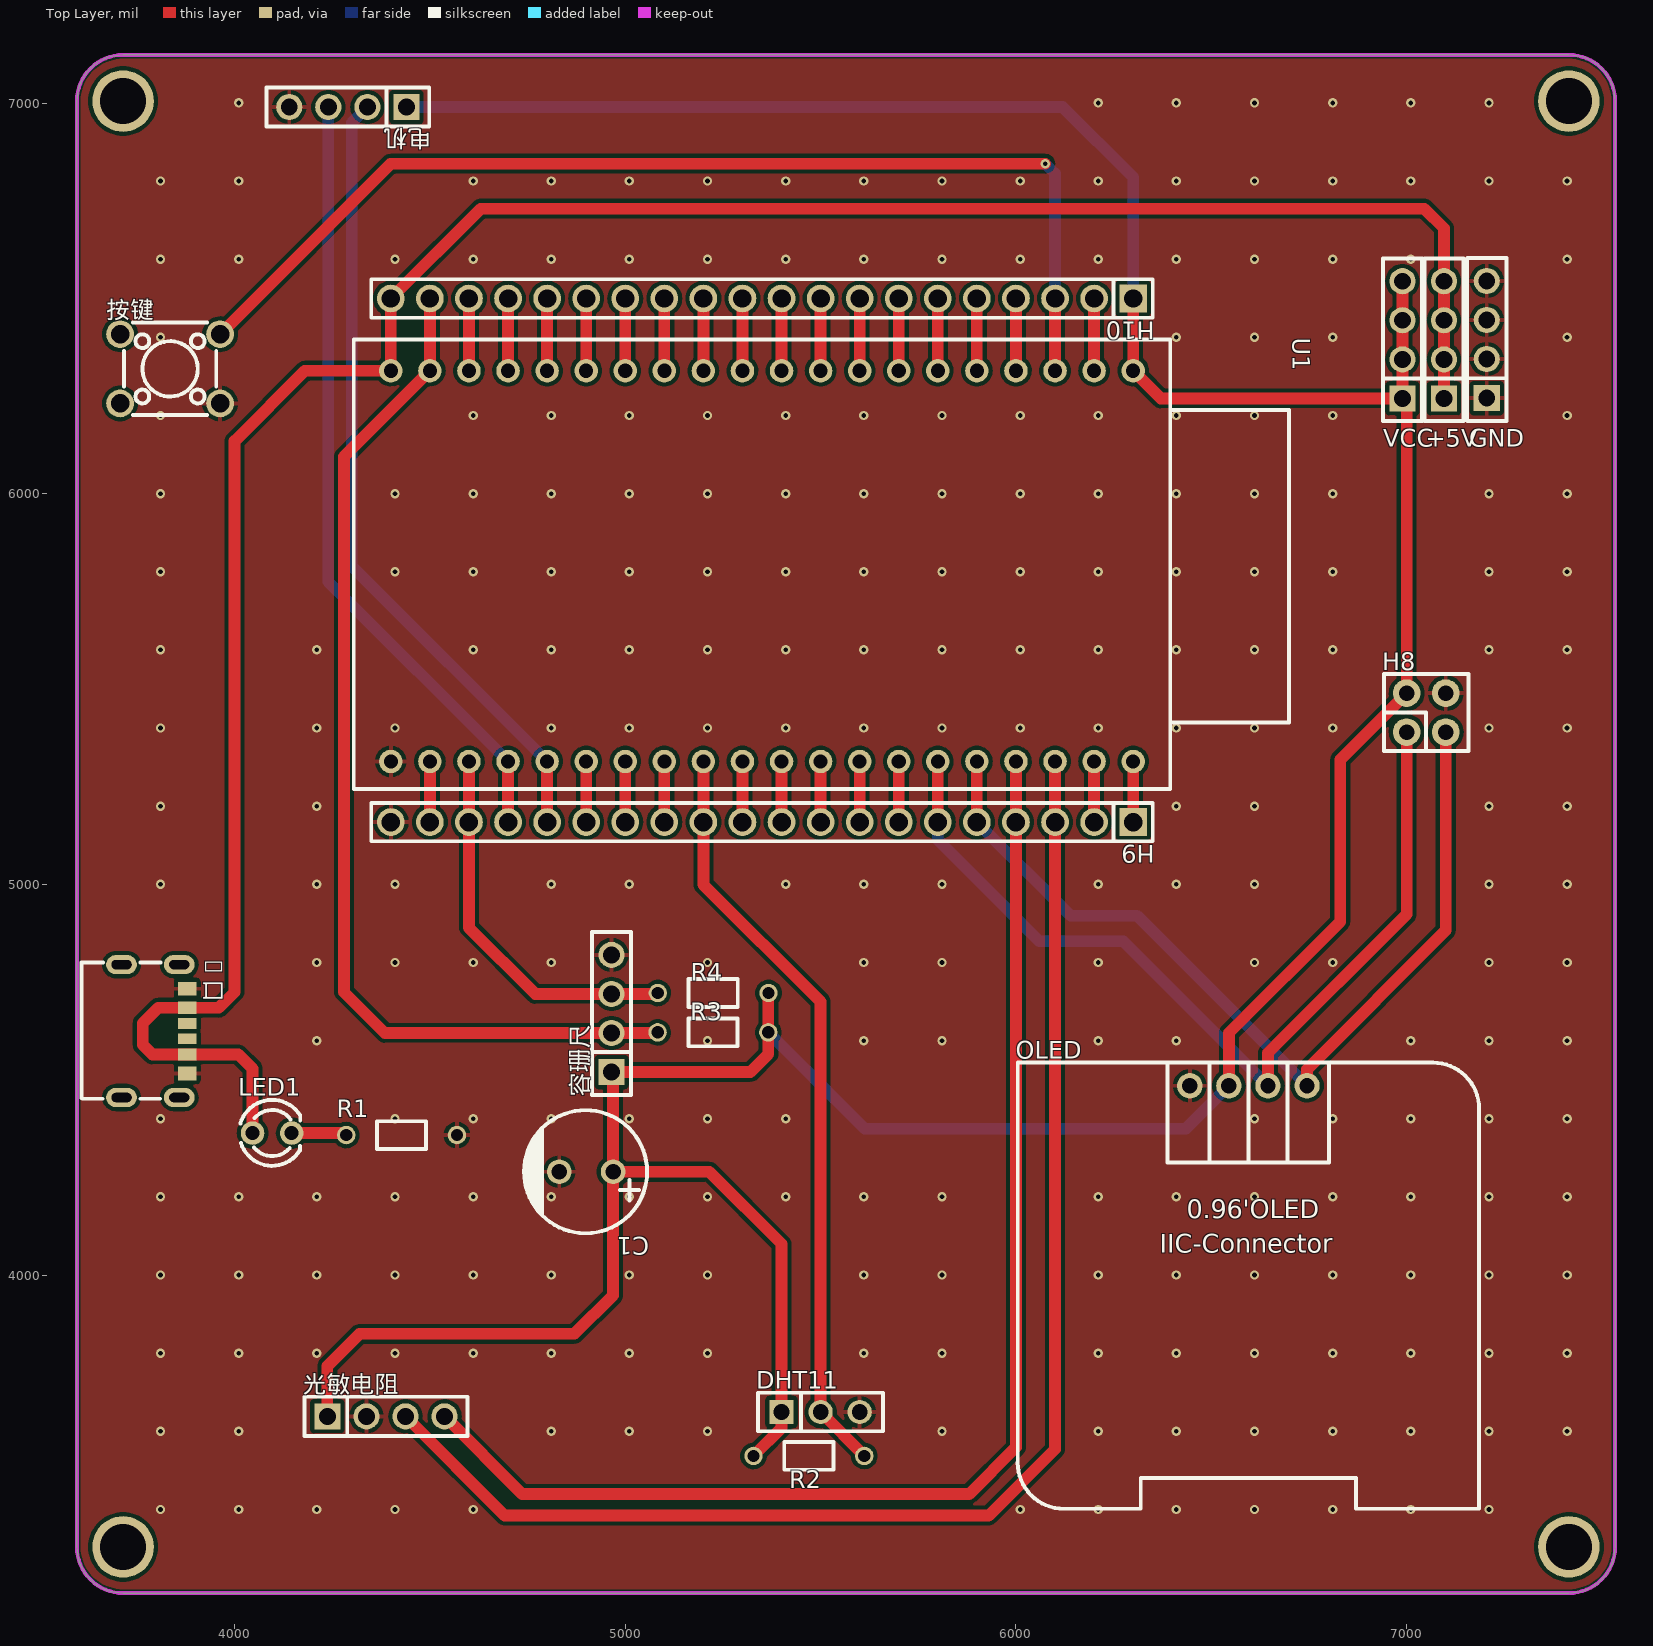
[diagram p0: Top Layer view]
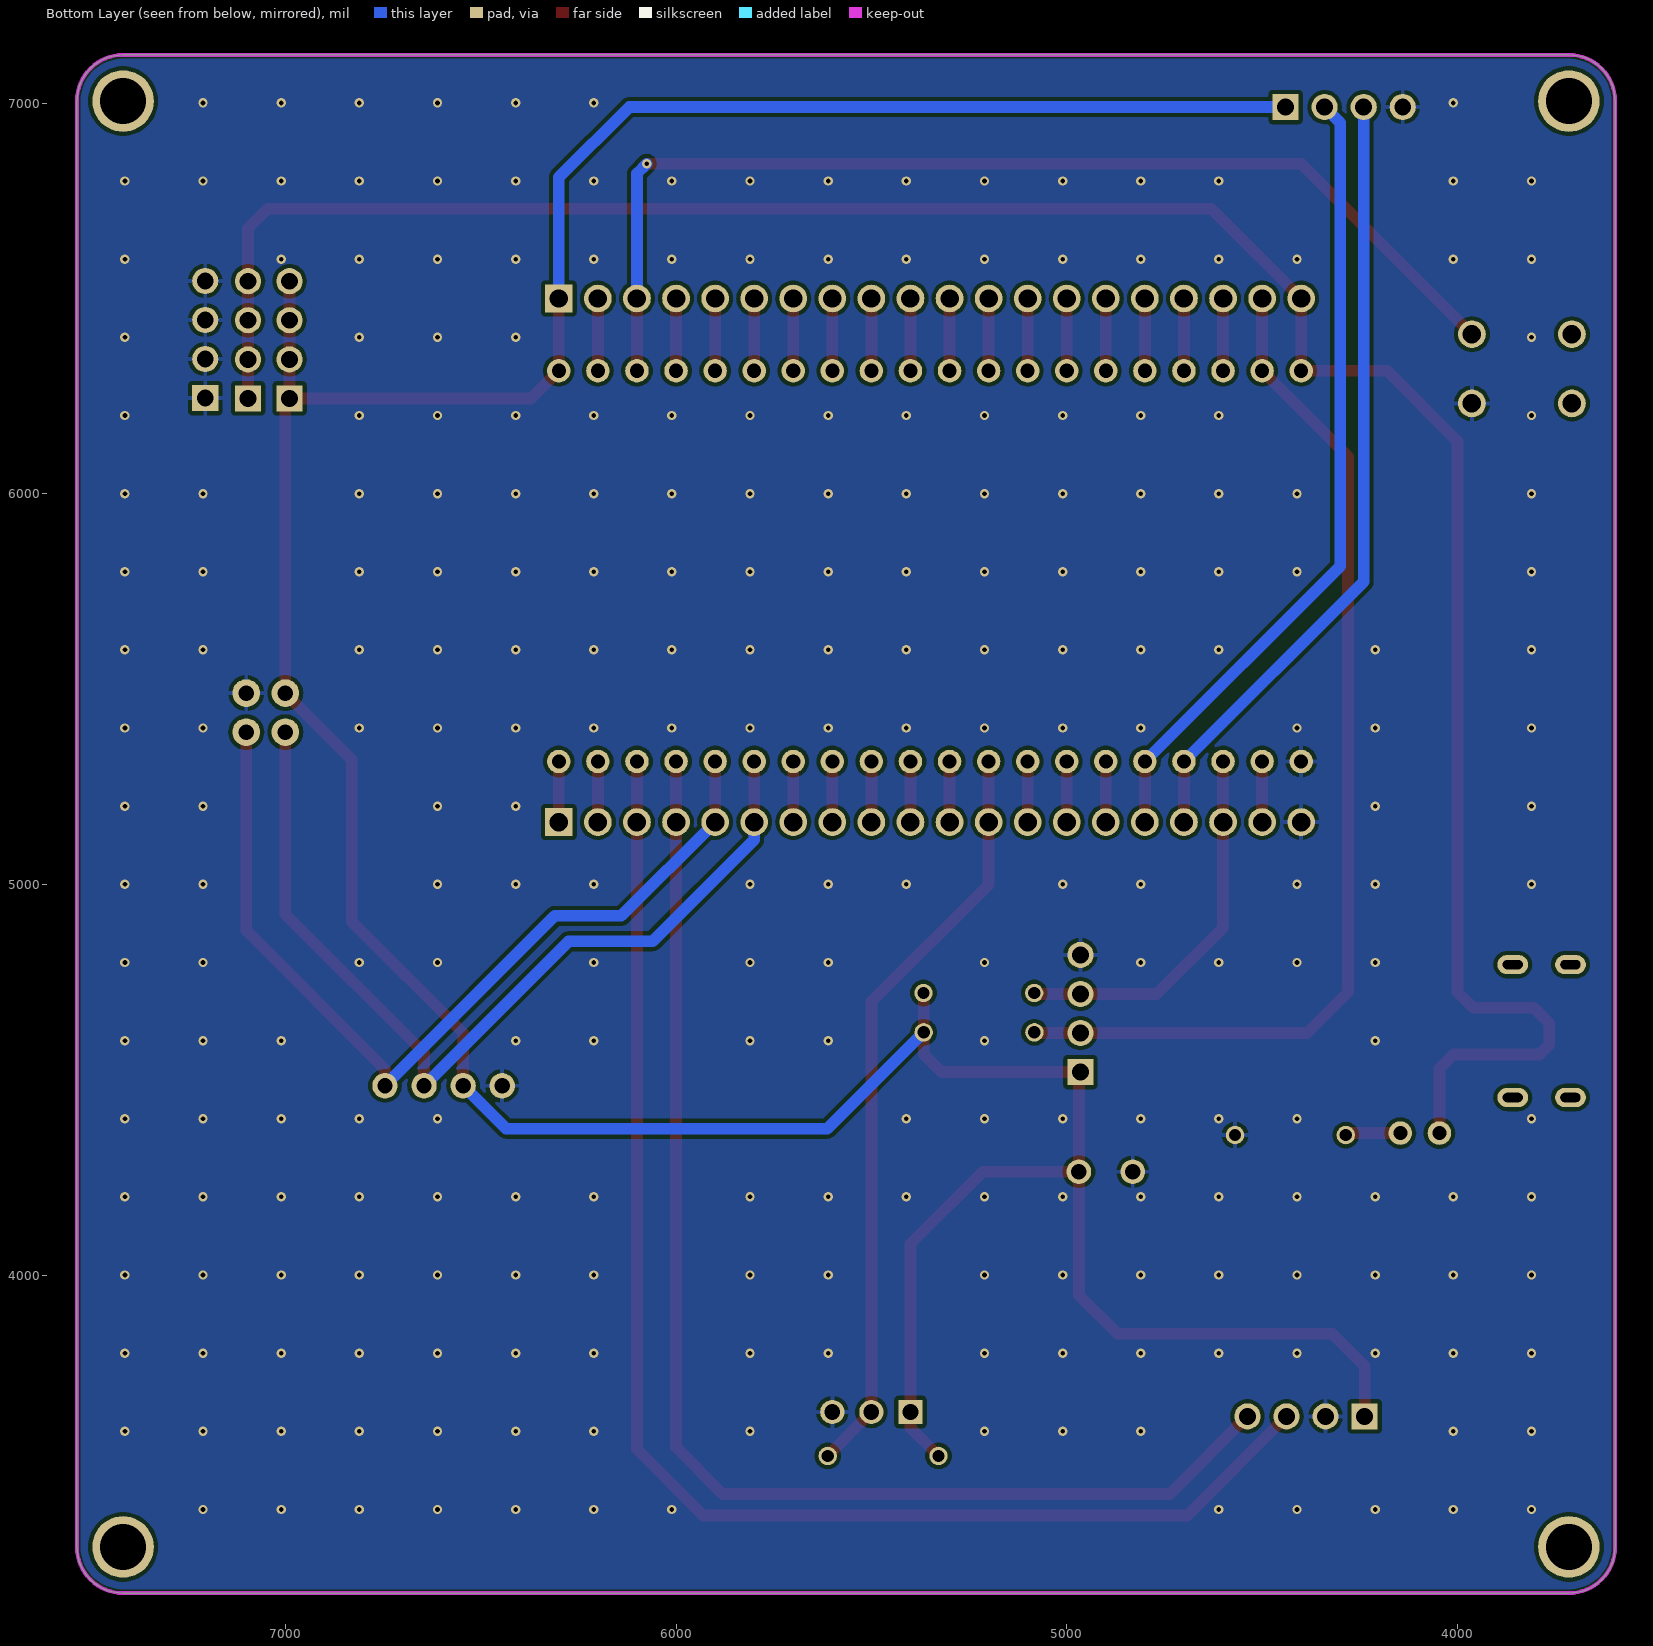
[diagram p1: Bottom Layer view, seen from below]
# Altium PCB MISC51152.pcbdoc
Units mil, origin at the board's own origin, x right, y up, seen from the top; angles counter-clockwise.
Board outline 3937.01 x 3937.01 mil, 2 copper layers (Top Layer, Bottom Layer), stack 62.206 mil thick; 20 components, 41 nets, 145 pads, 254 vias.

## Layer stack, top to bottom
Top Solder Mask Layer: solder mask 0.394, Dk 3.3
Top Layer: signal copper 1.379
Dielectric1: surface 59.449, FR4, Dk 4.5
Bottom Layer: signal copper 1.378
Bottom Solder Mask Layer: solder mask 0.394, Dk 3.3

## Board outline
3714.61,7123.5 ccw(c3714.61,7005.39) 3596.5,7005.39 3596.5,3304.61 ccw(c3714.61,3304.61) 3714.61,3186.5 7415.39,3186.5 ccw(c7415.39,3304.61) 7533.5,3304.61 7533.5,7005.39 ccw(c7415.39,7005.39) 7415.39,7123.5 3714.61,7123.5

## Design rules (kind name [scope] priority, off if disabled: settings)
BoardOutlineClearance copperThickness2oz_1 [All] p2 off: genericclearance=7.99 ignorepadtopadclearanceinfootprint=FALSE except(0: Arc-SplitContinuation Track-SplitContinuation SMDPad-SplitContinuation THPad-SplitContinuation Via-SplitContinuation Fill-SplitContinuation Region-SplitContinuation Poly-SplitContinuation Text-SplitContinuation Hole-SplitContinuation; 5.98: Arc-CutoutEdge Track-CutoutEdge SMDPad-CutoutEdge THPad-CutoutEdge Via-CutoutEdge Text-CutoutEdge; 6.9: Hole-OutlineEdge Hole-CutoutEdge; 10: Poly-OutlineEdge Poly-CutoutEdge; 11.81: Arc-OutlineEdge Track-OutlineEdge SMDPad-OutlineEdge THPad-OutlineEdge Via-OutlineEdge Fill-OutlineEdge Region-OutlineEdge Text-OutlineEdge Fill-CutoutEdge Region-CutoutEdge)
BoardOutlineClearance Plane_innerPlane_1 [All] p4 off: genericclearance=4.02 ignorepadtopadclearanceinfootprint=FALSE except(0: Arc-SplitContinuation Track-SplitContinuation SMDPad-SplitContinuation THPad-SplitContinuation Via-SplitContinuation Fill-SplitContinuation Region-SplitContinuation Poly-SplitContinuation Text-SplitContinuation Hole-SplitContinuation; 5.98: Arc-CutoutEdge Track-CutoutEdge SMDPad-CutoutEdge THPad-CutoutEdge Via-CutoutEdge Text-CutoutEdge; 6.9: Hole-OutlineEdge Hole-CutoutEdge; 10: Poly-OutlineEdge Poly-CutoutEdge; 11.81: Arc-OutlineEdge Track-OutlineEdge SMDPad-OutlineEdge THPad-OutlineEdge Via-OutlineEdge Fill-OutlineEdge Region-OutlineEdge Text-OutlineEdge Fill-CutoutEdge Region-CutoutEdge)
BoardOutlineClearance Copper_copperRegion_1 [All] p6 off: genericclearance=4.02 ignorepadtopadclearanceinfootprint=FALSE except(0: Arc-SplitContinuation Track-SplitContinuation SMDPad-SplitContinuation THPad-SplitContinuation Via-SplitContinuation Fill-SplitContinuation Region-SplitContinuation Poly-SplitContinuation Text-SplitContinuation Hole-SplitContinuation; 5.98: Arc-CutoutEdge Track-CutoutEdge SMDPad-CutoutEdge THPad-CutoutEdge Via-CutoutEdge Text-CutoutEdge; 6.9: Hole-OutlineEdge Hole-CutoutEdge; 10: Poly-OutlineEdge Poly-CutoutEdge; 11.81: Arc-OutlineEdge Track-OutlineEdge SMDPad-OutlineEdge THPad-OutlineEdge Via-OutlineEdge Fill-OutlineEdge Region-OutlineEdge Text-OutlineEdge Fill-CutoutEdge Region-CutoutEdge)
BoardOutlineClearance Copper_copperRegion_copperThickness1oz_1 [All] p8 off: genericclearance=4.02 ignorepadtopadclearanceinfootprint=FALSE except(0: Arc-SplitContinuation Track-SplitContinuation SMDPad-SplitContinuation THPad-SplitContinuation Via-SplitContinuation Fill-SplitContinuation Region-SplitContinuation Poly-SplitContinuation Text-SplitContinuation Hole-SplitContinuation; 5.98: Arc-CutoutEdge Track-CutoutEdge SMDPad-CutoutEdge THPad-CutoutEdge Via-CutoutEdge Text-CutoutEdge; 6.9: Hole-OutlineEdge Hole-CutoutEdge; 10: Poly-OutlineEdge Poly-CutoutEdge; 11.81: Arc-OutlineEdge Track-OutlineEdge SMDPad-OutlineEdge THPad-OutlineEdge Via-OutlineEdge Fill-OutlineEdge Region-OutlineEdge Text-OutlineEdge Fill-CutoutEdge Region-CutoutEdge)
BoardOutlineClearance Copper_copperRegion_Copper_copperRegion_1 [All] p10 off: genericclearance=4.02 ignorepadtopadclearanceinfootprint=FALSE except(0: Arc-SplitContinuation Track-SplitContinuation SMDPad-SplitContinuation THPad-SplitContinuation Via-SplitContinuation Fill-SplitContinuation Region-SplitContinuation Poly-SplitContinuation Text-SplitContinuation Hole-SplitContinuation; 5.98: Arc-CutoutEdge Track-CutoutEdge SMDPad-CutoutEdge THPad-CutoutEdge Via-CutoutEdge Text-CutoutEdge; 6.9: Hole-OutlineEdge Hole-CutoutEdge; 10: Poly-OutlineEdge Poly-CutoutEdge; 11.81: Arc-OutlineEdge Track-OutlineEdge SMDPad-OutlineEdge THPad-OutlineEdge Via-OutlineEdge Fill-OutlineEdge Region-OutlineEdge Text-OutlineEdge Fill-CutoutEdge Region-CutoutEdge)
BoardOutlineClearance copperThickness1oz_1 [All] p12: genericclearance=4.02 ignorepadtopadclearanceinfootprint=FALSE except(0: Arc-SplitContinuation Track-SplitContinuation SMDPad-SplitContinuation THPad-SplitContinuation Via-SplitContinuation Fill-SplitContinuation Region-SplitContinuation Poly-SplitContinuation Text-SplitContinuation Hole-SplitContinuation; 5.98: Arc-CutoutEdge Track-CutoutEdge SMDPad-CutoutEdge THPad-CutoutEdge Via-CutoutEdge Text-CutoutEdge; 6.9: Hole-OutlineEdge Hole-CutoutEdge; 10: Poly-OutlineEdge Poly-CutoutEdge; 11.81: Arc-OutlineEdge Track-OutlineEdge SMDPad-OutlineEdge THPad-OutlineEdge Via-OutlineEdge Fill-OutlineEdge Region-OutlineEdge Text-OutlineEdge Fill-CutoutEdge Region-CutoutEdge)
Clearance copperThickness2oz [All] p1 off: gap=7.99 ignorepadtopadclearanceinfootprint=FALSE except(5.98: SMDPad-Track SMDPad-SMDPad THPad-Track SMDPad-THPad THPad-THPad Track-Via SMDPad-Via THPad-Via Via-Via Fill-SMDPad Region-SMDPad Fill-THPad Region-THPad Fill-Via Region-Via Fill-Fill Fill-Region Region-Region Arc-Track Arc-SMDPad Arc-THPad Arc-Via Fill-Arc Region-Arc Arc-Arc Text-Track SMDPad-Text Text-THPad Text-Via Fill-Text Region-Text Arc-Text Text-Text; 6.9: Hole-Track Hole-SMDPad Hole-THPad Hole-Via Fill-Hole Region-Hole Hole-Arc Hole-Text; 10: Poly-Track Poly-SMDPad Poly-THPad Poly-Via Poly-Fill Poly-Region Poly-Poly Poly-Arc Poly-Text Poly-Hole; 11.81: Fill-Track Region-Track)
Clearance Plane_innerPlane [All] p3 off: gap=4.02 ignorepadtopadclearanceinfootprint=FALSE except(5.98: SMDPad-Track SMDPad-SMDPad THPad-Track SMDPad-THPad THPad-THPad Track-Via SMDPad-Via THPad-Via Via-Via Fill-SMDPad Region-SMDPad Fill-THPad Region-THPad Fill-Via Region-Via Fill-Fill Fill-Region Region-Region Arc-Track Arc-SMDPad Arc-THPad Arc-Via Fill-Arc Region-Arc Arc-Arc Text-Track SMDPad-Text Text-THPad Text-Via Fill-Text Region-Text Arc-Text Text-Text; 6.9: Hole-Track Hole-SMDPad Hole-THPad Hole-Via Fill-Hole Region-Hole Hole-Arc Hole-Text; 10: Poly-Track Poly-SMDPad Poly-THPad Poly-Via Poly-Fill Poly-Region Poly-Poly Poly-Arc Poly-Text Poly-Hole; 11.81: Fill-Track Region-Track)
Clearance Copper_copperRegion [All] p5 off: gap=4.02 ignorepadtopadclearanceinfootprint=FALSE except(5.98: SMDPad-Track SMDPad-SMDPad THPad-Track SMDPad-THPad THPad-THPad Track-Via SMDPad-Via THPad-Via Via-Via Fill-SMDPad Region-SMDPad Fill-THPad Region-THPad Fill-Via Region-Via Fill-Fill Fill-Region Region-Region Arc-Track Arc-SMDPad Arc-THPad Arc-Via Fill-Arc Region-Arc Arc-Arc Text-Track SMDPad-Text Text-THPad Text-Via Fill-Text Region-Text Arc-Text Text-Text; 6.9: Hole-Track Hole-SMDPad Hole-THPad Hole-Via Fill-Hole Region-Hole Hole-Arc Hole-Text; 10: Poly-Track Poly-SMDPad Poly-THPad Poly-Via Poly-Fill Poly-Region Poly-Poly Poly-Arc Poly-Text Poly-Hole; 11.81: Fill-Track Region-Track)
Clearance Copper_copperRegion_copperThickness1oz [All] p7 off: gap=4.02 ignorepadtopadclearanceinfootprint=FALSE except(5.98: SMDPad-Track SMDPad-SMDPad THPad-Track SMDPad-THPad THPad-THPad Track-Via SMDPad-Via THPad-Via Via-Via Fill-SMDPad Region-SMDPad Fill-THPad Region-THPad Fill-Via Region-Via Fill-Fill Fill-Region Region-Region Arc-Track Arc-SMDPad Arc-THPad Arc-Via Fill-Arc Region-Arc Arc-Arc Text-Track SMDPad-Text Text-THPad Text-Via Fill-Text Region-Text Arc-Text Text-Text; 6.9: Hole-Track Hole-SMDPad Hole-THPad Hole-Via Fill-Hole Region-Hole Hole-Arc Hole-Text; 10: Poly-Track Poly-SMDPad Poly-THPad Poly-Via Poly-Fill Poly-Region Poly-Poly Poly-Arc Poly-Text Poly-Hole; 11.81: Fill-Track Region-Track)
Clearance Copper_copperRegion_Copper_copperRegion [All] p9 off: gap=4.02 ignorepadtopadclearanceinfootprint=FALSE except(5.98: SMDPad-Track SMDPad-SMDPad THPad-Track SMDPad-THPad THPad-THPad Track-Via SMDPad-Via THPad-Via Via-Via Fill-SMDPad Region-SMDPad Fill-THPad Region-THPad Fill-Via Region-Via Fill-Fill Fill-Region Region-Region Arc-Track Arc-SMDPad Arc-THPad Arc-Via Fill-Arc Region-Arc Arc-Arc Text-Track SMDPad-Text Text-THPad Text-Via Fill-Text Region-Text Arc-Text Text-Text; 6.9: Hole-Track Hole-SMDPad Hole-THPad Hole-Via Fill-Hole Region-Hole Hole-Arc Hole-Text; 10: Poly-Track Poly-SMDPad Poly-THPad Poly-Via Poly-Fill Poly-Region Poly-Poly Poly-Arc Poly-Text Poly-Hole; 11.81: Fill-Track Region-Track)
Clearance copperThickness1oz [All] p11: gap=4.02 ignorepadtopadclearanceinfootprint=FALSE except(5.98: SMDPad-Track SMDPad-SMDPad THPad-Track SMDPad-THPad THPad-THPad Track-Via SMDPad-Via THPad-Via Via-Via Fill-SMDPad Region-SMDPad Fill-THPad Region-THPad Fill-Via Region-Via Fill-Fill Fill-Region Region-Region Arc-Track Arc-SMDPad Arc-THPad Arc-Via Fill-Arc Region-Arc Arc-Arc Text-Track SMDPad-Text Text-THPad Text-Via Fill-Text Region-Text Arc-Text Text-Text; 6.9: Hole-Track Hole-SMDPad Hole-THPad Hole-Via Fill-Hole Region-Hole Hole-Arc Hole-Text; 10: Poly-Track Poly-SMDPad Poly-THPad Poly-Via Poly-Fill Poly-Region Poly-Poly Poly-Arc Poly-Text Poly-Hole; 11.81: Fill-Track Region-Track)
DiffPairsRouting differentialPair [All] p1: maxlimit=6 minlimit=6 mostfreqgap=6 toplayer_minwidth=5 toplayer_prefwidth=10 toplayer_maxwidth=100 toplayer_mingap=6 toplayer_prefgap=6 toplayer_maxgap=6 bottomlayer_minwidth=5 bottomlayer_prefwidth=10 bottomlayer_maxwidth=100 bottomlayer_mingap=6 bottomlayer_prefgap=6 bottomlayer_maxgap=6 maxuncoupledlength=10
HoleToHoleClearance otherClearance [All] p1: gap=11.81 allowstackedmicrovias=TRUE
Length netLength [All] p1: minlimit=0 maxlimit=0
PasteMaskExpansion pasteMaskExpansion [All] p1: expansion=0
PlaneConnect innerPlane [All] p1: planeconnectstyle=Relief reliefexpansion=20 reliefentries=4 reliefconductorwidth=10 reliefairgap=10
PolygonConnect copperRegion_copperThickness1oz [All] p1 off: connectstyle=Relief reliefconductorwidth=10 reliefentries=4 polygonreliefangle="90 Angle" airgapwidth=10 via.connectstyle=Relief via.reliefconductorwidth=10 via.reliefentries=4 via.polygonreliefangle="90 Angle" via.airgapwidth=10
PolygonConnect copperRegion_Copper_copperRegion [All] p2 off: connectstyle=Relief reliefconductorwidth=10 reliefentries=4 polygonreliefangle="90 Angle" airgapwidth=10 via.connectstyle=Relief via.reliefconductorwidth=10 via.reliefentries=4 via.polygonreliefangle="90 Angle" via.airgapwidth=10
PolygonConnect copperRegion [All] p3: connectstyle=Relief reliefconductorwidth=10 reliefentries=4 polygonreliefangle="90 Angle" airgapwidth=10 via.connectstyle=Relief via.reliefconductorwidth=10 via.reliefentries=4 via.polygonreliefangle="90 Angle" via.airgapwidth=10
RoutingVias viaSize [All] p1: holewidth=12.01 width=24.02 viastyle="Through Hole" minholewidth=11.81 minwidth=19.68 maxholewidth=248.03 maxwidth=393.7
SolderMaskExpansion solderMaskExpansion [IsVia] p1: expansion=-1000 istentingtop=TRUE
SolderMaskExpansion solderMaskExpansion [All] p2: expansion=2 istentingtop=FALSE
Width copperThickness2oz_2 [All] p1 off: maxlimit=100 minlimit=8 preferedwidth=10
Width copperThickness1oz_2 [All] p2: maxlimit=100 minlimit=5 preferedwidth=10

## Components (designator, comment, footprint, x,y, rotation, side; value= is the part's Value field where it differs from the comment)
+5V "" HDR-TH_4P-P2.54-V-F 7095.49,6394.24 r90 top
C1 "100uF" CAP-TH_BD8.0-P3.50-D0.6-FD_1 4900,4265 r180 top
C口 "" "USB_ TYPE-C-6P" 3795,4630 r270 top
DHT11 "" HDR-TH_3P-P2.54-V-F 5500,3650 r0 top
GND "" HDR-TH_4P-P2.54-V-F 7205,6395 r90 top
H8 "" HDR-TH_4P-P2.54-V-F-R2-C2-S2.54 7050,5440 r0 top
H9 "" HDR-TH_20P-P2.54-V-M-1 5350,5160 r180 top
H10 "" HDR-TH_20P-P2.54-V-M-1 5350,6500 r180 top
LED1 "" LED_TH-3mm 4096.16,4363.96 r0 top
OLED "" 0.96OLED_4P 6595,4485 r0 top
R1 "220Ω" Res_1/8W 4427.54,4356.32 r0 top
R2 "4.7K" Res_1/8W 5470,3540 r180 top
R3 "4.7K" Res_1/8W 5224.49,4619.19 r0 top
R4 "4.7K" Res_1/8W 5225,4720 r0 top
U1 "" ESP32-S3-CAM 4400,6315 r270 top
VCC "" HDR-TH_4P-P2.54-V-F 6989.27,6394.24 r90 top
光敏电阻 "" HDR-TH_4P-P2.54-V-F 4387.54,3638.97 r0 top
容珊尺 "" HDR-TH_4P-P2.54-V-F 4965,4670 r90 top
按键 "" SW-TH_4P-L6.0-W6.0-P4.50-LS6.5 3835,6320 r0 top
电机 "" HDR-TH_4P-P2.54-V-F 4290,6990 r180 top

## Footprints (in the part's own frame and the unit in brackets; to place one, negate y for a bottom-side part, rotate by r counter-clockwise, add the part's x,y. Pads: shape width x height; smd on the part's side, far side on the other; paste and mask are expansions set on the pad)
0.96OLED_4P [mm]
  round 1.65 hole 1 copper offset 0,0: 1(-3.81,-0.001) 2(-1.27,0.002) 3(1.27,0.002) 4(3.81,0.002)
  silkscreen extent -15,-27.5 15,1.5
CAP-TH_BD8.0-P3.50-D0.6-FD_1 [mm]
  round 1.6 hole 1: 1(-1.75,0) 2(1.75,0)
  silkscreen extent -3.96,-4 4.04,4
ESP32-S3-CAM [mil]
  round 60 hole 36: 1(0,1900) 2(0,1800) 3(0,1700) 4(0,1600) 5(0,1500) 6(0,1400) 7(0,1300) 8(0,1200) 9(0,1100) 10(0,1000) 11(0,900) 12(0,800) 13(0,700) 14(0,600) 15(0,500) 16(0,400) 17(0,300) 18(0,200) 19(0,100) 20(0,0) 21(1000,1900) 22(1000,1800) 23(1000,1700) 24(1000,1600) 25(1000,1500) 26(1000,1400) 27(1000,1300) 28(1000,1200) 29(1000,1100) 30(1000,1000) 31(1000,900) 32(1000,800) 33(1000,700) 34(1000,600) 35(1000,500) 36(1000,400) 37(1000,300) 38(1000,200) 39(1000,100) 40(1000,0)
  silkscreen extent -80,-95 1070,2299
HDR-TH_3P-P2.54-V-F [mil]
  rect 62x62 hole 40.16: 1(-100,0)
  round 62 hole 40.16: 2(0,0) 3(100,0)
  silkscreen extent -160,-49 160,49
HDR-TH_4P-P2.54-V-F [mm]
  rect 1.7x1.7 hole 1.1: 1(-3.81,0)
  round 1.7 hole 1.1: 2(-1.27,0) 3(1.27,0) 4(3.81,0)
  silkscreen extent -5.29,-1.27 5.29,1.27
HDR-TH_4P-P2.54-V-F-R2-C2-S2.54 [mm]
  round 1.8 hole 1: 1(-1.27,-1.27) 2(-1.27,1.27) 3(1.27,-1.27) 4(1.27,1.27)
  silkscreen extent -2.74,-2.5 2.74,2.5
HDR-TH_20P-P2.54-V-M-1 [mm]
  rect 1.8x1.8 hole 1.2: 1(-24.13,0)
  round 1.8 hole 1.2: 2(-21.59,0) 3(-19.05,0) 4(-16.51,0) 5(-13.97,0) 6(-11.43,0) 7(-8.89,0) 8(-6.35,0) 9(-3.81,0) 10(-1.27,0) 11(1.27,0) 12(3.81,0) 13(6.35,0) 14(8.89,0) 15(11.43,0) 16(13.97,0) 17(16.51,0) 18(19.05,0) 19(21.59,0) 20(24.13,0)
  silkscreen extent -25.4,-1.25 25.4,1.25
LED_TH-3mm [mil]
  round 60 hole 36 paste+0 mask+2: 1(-50,0) 2(50,0)
  silkscreen extent -81,-84 72,85
Res_1/8W [mil]
  round 47.2 hole 31.5 paste+0 mask+2: 1(-141.7,2.48) 2(141.7,2.48)
  silkscreen extent -63,-33 63,38
SW-TH_4P-L6.0-W6.0-P4.50-LS6.5 [mm]
  round 1.8 hole 1.2: 1(-3.25,2.25) 2(3.25,2.25) 3(-3.25,-2.25) 4(3.25,-2.25)
  silkscreen extent -3,-3 3,3
"USB_ TYPE-C-6P" [mm]
  oval 1.25x2 hole 0.6 slot 1.3 at 90 deg paste+0 mask+0.05: 7(-4.193,1.611) 8(4.447,1.611) 9(-4.193,-2.139) 10(4.447,-2.139)
  rect 0.7x1.2 smd paste-100 mask+0.05: A5(-0.373,2.139) B5(0.627,2.139)
  rect 0.8x1.2 smd paste-100 mask+0.05: A9(1.647,2.139) B9(-1.393,2.139)
  rect 0.9x1.2 smd paste-100 mask+0.05: A12(2.877,2.139) B12(-2.623,2.139)
  silkscreen extent -4.34,-4.75 4.52,0.39

## Free pads (board coordinates)
  round 157.48 hole 118.11: 1(3714.61,7005.39) 1(3714.61,3304.61) 1(7415.39,7005.39) 1(7415.39,3304.61)

## Via types
v1: diameter 24.02, hole 12, Top Layer to Bottom Layer, 254 vias

## Nets (pads, with @x,y where several pads share a name; then routed paths per layer and width w, separated by ;. In a path a pad name is that pad's centre, name@x,y a point inside that pad or via, vN(x,y) a via of type N, cw(c..) or ccw(c..) an arc to the next point about the centre after c; other vN are vias at no path point)
0: H9.13 U1.33 | length 160
  Top Layer w30: H9.13@5100,5155 U1.33
1: H9.3 U1.23 光敏电阻.3 | length 3598.1
  Top Layer w30: 光敏电阻.3 4691.51,3385 5930,3385 6100,3555 H9.3 U1.23
2: H9.4 U1.24 光敏电阻.4 | length 3349.6
  Top Layer w30: 光敏电阻.4 4736.51,3440 5880,3440 6000,3560 H9.4 U1.24
3: H10.12 U1.12 | length 185
  Top Layer w30: U1.12 H10.12
4: H10.3 U1.3 按键.2 | length 2833.2
  Top Layer w30: 按键.2 4399.37,6845 v1(6075,6845) ; U1.3 H10.3
  Bottom Layer w30: v1(6075,6845) 6100,6820 H10.3
5: H10.4 U1.4 | length 185
  Top Layer w30: U1.4 H10.4
6: H10.5 U1.5 | length 185
  Top Layer w30: U1.5 H10.5
7: H10.6 U1.6 | length 185
  Top Layer w30: U1.6 H10.6
8: H10.11 U1.11 | length 185
  Top Layer w30: U1.11 H10.11
9: H10.14 U1.14 | length 185
  Top Layer w30: U1.14 H10.14
10: H10.15 U1.15 | length 185
  Top Layer w30: U1.15 H10.15
11: H10.16 U1.16 | length 185
  Top Layer w30: U1.16 H10.16
12: H10.17 U1.17 | length 185
  Top Layer w30: U1.17 H10.17
13: H10.18 U1.18 | length 185
  Top Layer w30: U1.18 H10.18
14: H10.19 R3.1 U1.19 容珊尺.2 | length 2713.1
  Top Layer w30: H10.19 U1.19 4280,6095 4280,4725 4385,4620 容珊尺.2 5081.12,4620 R3.1
15: H10.7 U1.7 | length 185
  Top Layer w30: U1.7 H10.7
16: H10.8 U1.8 | length 185
  Top Layer w30: U1.8 H10.8
17: H10.9 U1.9 | length 185
  Top Layer w30: U1.9 H10.9
18: H10.10 U1.10 | length 185
  Top Layer w30: U1.10 H10.10
19: H9.19 U1.39 | length 160
  Top Layer w30: H9.19@4500,5155 U1.39
20: H9.18 R4.1 U1.38 容珊尺.3 | length 979.7
  Top Layer w30: U1.38 H9.18 4600,4890 4770,4720 容珊尺.3 5080.82,4720 R4.1
21: H9.17 U1.37 电机.3 | length 2025.5
  Top Layer w30: H9.17@4700,5155 U1.37
  Bottom Layer w30: 电机.3 4240,5775 U1.37
35: DHT11.2 H9.12 R2.1 U1.32 | length 1948
  Top Layer w30: U1.32 H9.12 5200,5000 5500,4700 DHT11.2 5611.7,3538.3 R2.1
36: H9.11 U1.31 | length 160
  Top Layer w30: H9.11@5300,5155 U1.31
37: H9.10 U1.30 | length 160
  Top Layer w30: H9.10@5400,5155 U1.30
38: H9.9 U1.29 | length 160
  Top Layer w30: H9.9@5500,5155 U1.29
39: H9.8 U1.28 | length 160
  Top Layer w30: H9.8@5600,5155 U1.28
40: H9.7 U1.27 | length 160
  Top Layer w30: H9.7@5700,5155 U1.27
41: H8.1 H9.6 OLED.3 U1.26 | length 2362.9
  Top Layer w30: H9.6@5800,5155 U1.26 ; OLED.3@6645,4485.05 6645,4568.95 7000,4923.95 H8.1
  Bottom Layer w30: H9.6 5800,5115 6060,4855 6275.05,4855 OLED.3@6645,4485.05
42: H8.3 H9.5 OLED.4 U1.25 | length 2336.6
  Top Layer w30: H9.5@5900,5155 U1.25 ; OLED.4@6745,4485.05 6745,4527.53 7100,4882.53 H8.3
  Bottom Layer w30: H9.5 6140,4920 6310.05,4920 OLED.4@6745,4485.05
45: H9.14 U1.34 | length 160
  Top Layer w30: H9.14@5000,5155 U1.34
46: H10.13 U1.13 | length 185
  Top Layer w30: U1.13 H10.13
47: H9.16 U1.36 电机.2 | length 2058.7
  Top Layer w30: H9.16@4800,5155 U1.36
  Bottom Layer w30: 电机.2 4300,6950 4300,5815 U1.36
48: H9.15 U1.35 | length 160
  Top Layer w30: H9.15@4900,5155 U1.35
$1N17160: LED1.2 R1.1 | length 141.8
  Top Layer w30: LED1.2 4280.67,4363.96 R1.1
+5V: +5V.1 +5V.2 +5V.3 +5V.4 C口.A9 C口.B9 H10.20 LED1.1 U1.20 | length 6111
  Top Layer w30: LED1.1 4046.16,4528.84 4009.84,4565.16 C口.A9 3789.84,4565.16 3765,4590 3765,4645 3804.84,4684.84 C口.B9 3959.84,4684.84 4000,4725 4000,6135 4180,6315 U1.20 H10.20 4630,6730 7045,6730 7095.49,6679.51 +5V.4 +5V.3 +5V.2 +5V.1
GND: C1.2 C口.A12 C口.B12 DHT11.3 GND.1 GND.2 GND.3 GND.4 H8.4 H9.20 OLED.1 R1.2 U1.40 光敏电阻.2 容珊尺.4 按键.4 电机.4
  other v1: 3810.6,3400.6 4010.6,3400.6 4210.6,3400.6 4410.6,3400.6 4610.6,3400.6 6010.6,3400.6 6210.6,3400.6 6410.6,3400.6 6610.6,3400.6 6810.6,3400.6 7010.6,3400.6 7210.6,3400.6 3810.6,3600.6 4010.6,3600.6 4810.6,3600.6 5010.6,3600.6 5210.6,3600.6 5810.6,3600.6 6210.6,3600.6 6410.6,3600.6 6610.6,3600.6 6810.6,3600.6 7010.6,3600.6 7210.6,3600.6 7410.6,3600.6 3810.6,3800.6 4010.6,3800.6 4210.6,3800.6 4410.6,3800.6 4610.6,3800.6 4810.6,3800.6 5010.6,3800.6 5210.6,3800.6 5610.6,3800.6 5810.6,3800.6 6210.6,3800.6 6410.6,3800.6 6610.6,3800.6 6810.6,3800.6 7010.6,3800.6 7210.6,3800.6 7410.6,3800.6 3810.6,4000.6 4010.6,4000.6 4210.6,4000.6 4410.6,4000.6 4610.6,4000.6 4810.6,4000.6 5010.6,4000.6 5210.6,4000.6 5610.6,4000.6 5810.6,4000.6 6210.6,4000.6 6410.6,4000.6 6610.6,4000.6 6810.6,4000.6 7010.6,4000.6 7210.6,4000.6 7410.6,4000.6 3810.6,4200.6 4010.6,4200.6 4210.6,4200.6 4410.6,4200.6 4610.6,4200.6 4810.6,4200.6 5010.6,4200.6 5210.6,4200.6 5410.6,4200.6 5610.6,4200.6 5810.6,4200.6 6210.6,4200.6 6410.6,4200.6 6610.6,4200.6 6810.6,4200.6 7010.6,4200.6 7210.6,4200.6 7410.6,4200.6 3810.6,4400.6 4410.6,4400.6 4610.6,4400.6 4810.6,4400.6 5010.6,4400.6 5210.6,4400.6 5410.6,4400.6 6610.6,4400.6 6810.6,4400.6 7010.6,4400.6 7210.6,4400.6 7410.6,4400.6 4210.6,4600.6 5210.6,4600.6 5610.6,4600.6 5810.6,4600.6 6210.6,4600.6 6410.6,4600.6 7010.6,4600.6 7210.6,4600.6 7410.6,4600.6 4210.6,4800.6 4410.6,4800.6 4610.6,4800.6 4810.6,4800.6 5210.6,4800.6 5610.6,4800.6 5810.6,4800.6 6210.6,4800.6 6610.6,4800.6 6810.6,4800.6 7210.6,4800.6 7410.6,4800.6 3810.6,5000.6 4210.6,5000.6 4410.6,5000.6 4810.6,5000.6 5010.6,5000.6 5410.6,5000.6 5610.6,5000.6 5810.6,5000.6 6210.6,5000.6 6410.6,5000.6 6610.6,5000.6 7210.6,5000.6 7410.6,5000.6 3810.6,5200.6 4210.6,5200.6 6410.6,5200.6 6610.6,5200.6 7210.6,5200.6 7410.6,5200.6 3810.6,5400.6 4210.6,5400.6 4410.6,5400.6 4810.6,5400.6 5010.6,5400.6 5210.6,5400.6 5410.6,5400.6 5610.6,5400.6 5810.6,5400.6 6010.6,5400.6 6210.6,5400.6 6410.6,5400.6 6610.6,5400.6 6810.6,5400.6 7210.6,5400.6 7410.6,5400.6 3810.6,5600.6 4210.6,5600.6 4610.6,5600.6 4810.6,5600.6 5010.6,5600.6 5210.6,5600.6 5410.6,5600.6 5610.6,5600.6 5810.6,5600.6 6010.6,5600.6 6210.6,5600.6 6410.6,5600.6 6610.6,5600.6 6810.6,5600.6 7210.6,5600.6 7410.6,5600.6 3810.6,5800.6 4410.6,5800.6 4610.6,5800.6 4810.6,5800.6 5010.6,5800.6 5210.6,5800.6 5410.6,5800.6 5610.6,5800.6 5810.6,5800.6 6010.6,5800.6 6210.6,5800.6 6410.6,5800.6 6610.6,5800.6 6810.6,5800.6 7210.6,5800.6 7410.6,5800.6 3810.6,6000.6 4410.6,6000.6 4610.6,6000.6 4810.6,6000.6 5010.6,6000.6 5210.6,6000.6 5410.6,6000.6 5610.6,6000.6 5810.6,6000.6 6010.6,6000.6 6210.6,6000.6 6410.6,6000.6 6610.6,6000.6 6810.6,6000.6 7210.6,6000.6 7410.6,6000.6 3810.6,6200.6 4610.6,6200.6 4810.6,6200.6 5010.6,6200.6 5210.6,6200.6 5410.6,6200.6 5610.6,6200.6 5810.6,6200.6 6010.6,6200.6 6210.6,6200.6 6410.6,6200.6 6610.6,6200.6 6810.6,6200.6 7410.6,6200.6 3810.6,6400.6 6410.6,6400.6 6610.6,6400.6 6810.6,6400.6 7410.6,6400.6 3810.6,6600.6 4010.6,6600.6 4410.6,6600.6 4610.6,6600.6 4810.6,6600.6 5010.6,6600.6 5210.6,6600.6 5410.6,6600.6 5610.6,6600.6 5810.6,6600.6 6010.6,6600.6 6210.6,6600.6 6410.6,6600.6 6610.6,6600.6 6810.6,6600.6 7010.6,6600.6 7410.6,6600.6 3810.6,6800.6 4010.6,6800.6 4610.6,6800.6 4810.6,6800.6 5010.6,6800.6 5210.6,6800.6 5410.6,6800.6 5610.6,6800.6 5810.6,6800.6 6010.6,6800.6 6210.6,6800.6 6410.6,6800.6 6610.6,6800.6 6810.6,6800.6 7010.6,6800.6 7210.6,6800.6 7410.6,6800.6 4010.6,7000.6 6210.6,7000.6 6410.6,7000.6 6610.6,7000.6 6810.6,7000.6 7010.6,7000.6 7210.6,7000.6
RST: H10.2 U1.2 | length 185
  Top Layer w30: U1.2 H10.2
RX: H9.2 U1.22 | length 160
  Top Layer w30: H9.2@6200,5155 U1.22
TX: H9.1 U1.21 | length 160
  Top Layer w30: H9.1@6300,5155 U1.21
VCC: C1.1 DHT11.1 H8.2 H10.1 OLED.2 R2.2 R3.2 R4.2 U1.1 VCC.1 VCC.2 VCC.3 VCC.4 光敏电阻.1 容珊尺.1 电机.1 | length 9891.3
  Top Layer w30: 光敏电阻.1 4237.54,3767.54 4320,3850 4870,3850 4968.9,3948.9 C1.1 ; R2.2 5400,3609.22 DHT11.1 5400,4080 5215,4265 C1.1 ; R4.2 5366.19,4721.97 R3.2 5366.19,4566.19 5320,4520 容珊尺.1 4968.9,4516.1 C1.1 ; H10.1 U1.1 6370.76,6244.24 VCC.1 ; OLED.2@6545,4485.05 6545,4620 6830,4905 6830,5320 H8.2 7000,6233.51 VCC.1 ; VCC.4 VCC.3 VCC.2 VCC.1
  Bottom Layer w30: 电机.1 6120,6990 6300,6810 H10.1 ; R3.2 5612.86,4375 6434.95,4375 OLED.2@6545,4485.05
pads on no net: C口.7 C口.8 C口.9 C口.10 C口.A5 C口.B5 按键.1 按键.3

## Polygon pours and split planes (outlines as drawn)
GND on Bottom Layer (solid, remove dead copper, pour order 2): 3525,7245 3525,3080 7700,3080 7700,7245
GND on Top Layer (solid, remove dead copper, pour order 2): 3000,7415 3000,3000 7930,3000 7930,7415

## Keep-outs
Board Outline Layer:
  the board outline again, w10